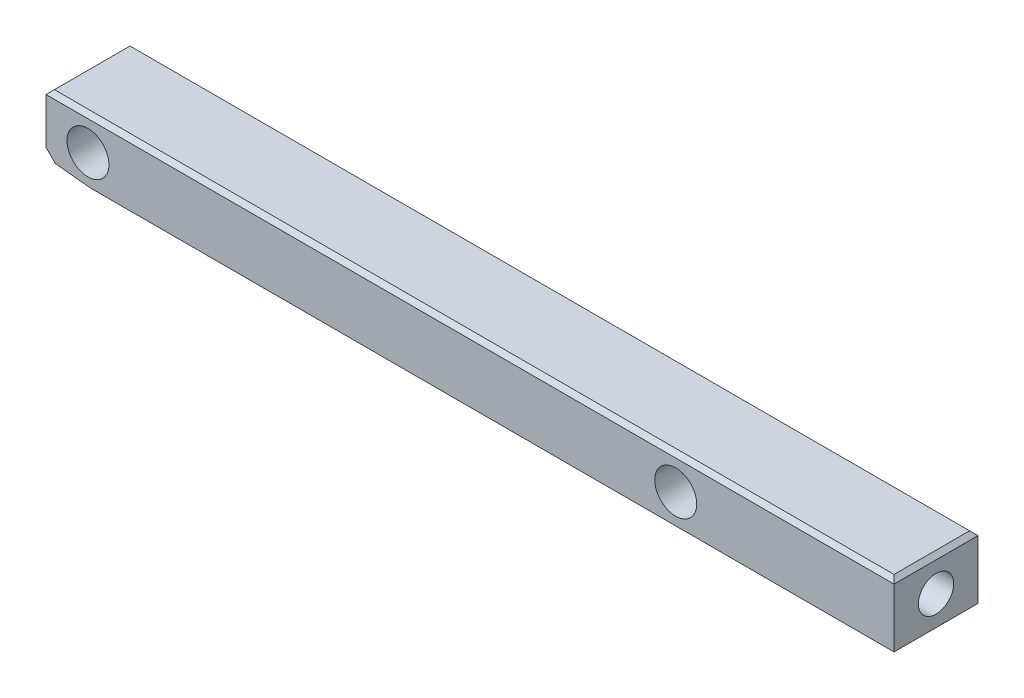
SolidWorks part; units mm, degrees
material "45"
ref_plane "Front Plane" through (0, 0, 0) normal (0, 0, 1) x (1, 0, 0)
ref_plane "Top Plane" through (0, 0, 0) normal (0, 1, 0) x (1, 0, 0)
ref_plane "Right Plane" through (0, 0, 0) normal (1, 0, 0) x (0, 0, -1)
sketch "Sketch1" plane through (0, 0, 0) normal (0, 0, 1) x (1, 0, 0)
  line L0 (-40.5, -4) -> (-50.5, -2.949)
  line L1 (-50.5, 4) -> (50.5, 4)
  line L2 (-50.5, 4) -> (-50.5, -2.949)
  line L3 (-40.5, -4) -> (50.5, -4)
  line L4 (50.5, 4) -> (50.5, -4)
  line L5 (-50.5, 4) -> (50.5, -4) construction
  line L6 (-49.5063, -3.9213) -> (50.5, 4) construction
  point P0 (0, 0)
  dimension "D1" = 101
  dimension "D2" = 8
  dimension "D3" = 174
  dimension "D4" = 10
  dimension "D5" = 4
extrude "Boss-Extrude1" add sketch "Sketch1" along normal mid plane 10
sketch "Sketch2" plane through (0, 0, 5) normal (0, 0, 1) x (1, 0, 0)
  line L0 (50.5, 4) -> (-50.5, 4) construction
  line L1 (-50.5, 4) -> (-50.5, -2.949) construction
  circle A0 centre (-45.5, 0) radius 2.5
  circle A1 centre (24.5, 0) radius 2.5
  dimension "D3" = 5
  dimension "D4" = 5
  dimension "D5" = 5
  dimension "D1" = 4
  dimension "D2" = 70
extrude "Cut-Extrude1" cut sketch "Sketch2" against normal through all
chamfer "Chamfer1" distance 0.5 angle 45 7 edges at (-50.5, 4, 0) (50.5, 4, 0) (50.5, -4, 0) (0, 4, -5) (0, 4, 5) (5, -4, -5) (5, -4, 5)
chamfer "Chamfer2" distance 1 angle 45 1 edges at (-50.5, -2.949, 0)
hole_wizard "M5 Tapped Hole1" positions "Sketch4" profile "Sketch3" tap size "M5" standard "Gb"
sketch "Sketch4" plane through (50.5, 0, 0) normal (1, 0, 0) x (0, 0, -1)
  line L0 (4.5, -4) -> (-4.5, -4) construction
  line L1 (-5, -3.5) -> (-5, 3.5) construction
  point P0 (0, 0)
  dimension "D1" = 4
  dimension "D2" = 5
sketch "Sketch3" plane through (50.5, 0, 0) normal (0, 1, 0) x (0, 0, -1)
  line L0 (0, 0) -> (0, 27.2618)
  line L1 (0, 27.2618) -> (2.1, 26)
  line L2 (2.1, 26) -> (2.1, 0)
  line L5 (2.1, 0) -> (0, 0)
  line L10 (0, 27.2618) -> (-2.1, 26) construction
  line L11 (0, -6.35) -> (0, 107.95) construction
  dimension "螺纹孔钻头直径" = 4.2
  dimension "螺纹孔钻头深度" = 26
  dimension "导头角度" = 118
cosmetic thread "Hole cosmetic thread 1" parameters "D1"=24, "D2"=5
